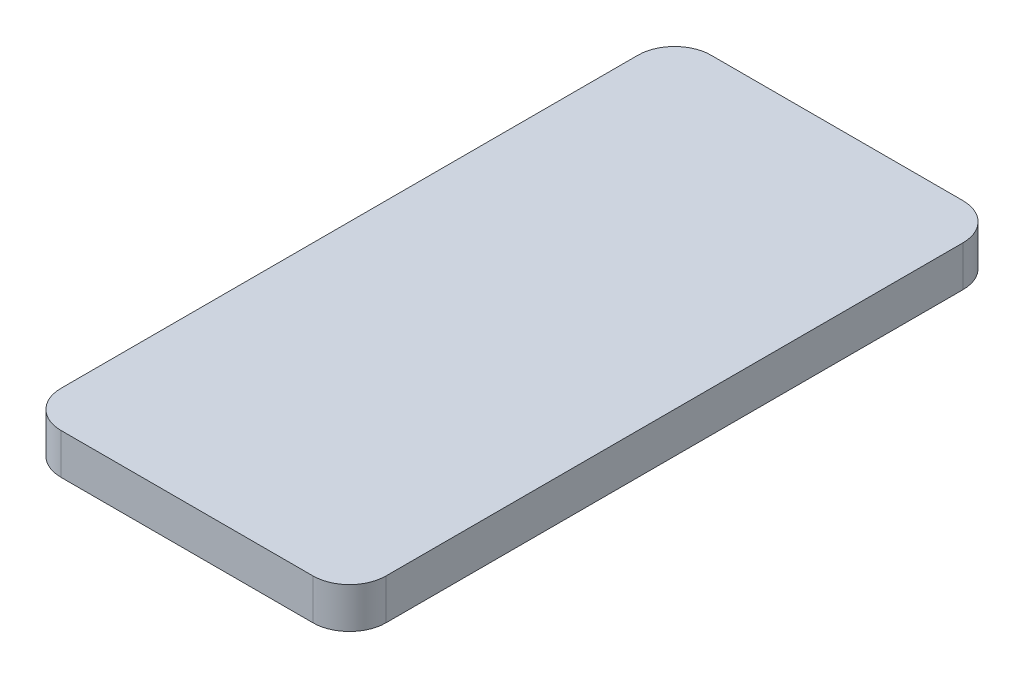
from build123d import *

# Parameters (mm, degrees)
SKETCH_1_W      = 40
SKETCH_1_H      = 80
EXTRUDE_1_DEPTH = 2.5
FILLET_1_R      = 4.5


with BuildPart() as part:
    # 草图1 → 凸台-拉伸1 (new, symmetric)
    with BuildSketch(Plane(origin=(0, 0, 0), x_dir=(1, 0, 0), z_dir=(0, 1, 0))):
        Rectangle(SKETCH_1_W, SKETCH_1_H)
    extrude(amount=EXTRUDE_1_DEPTH, both=True)

    # 圆角1
    fillet_1_edges = [part.edges().sort_by_distance(p)[0] for p in [
        (20, 0, 40),
        (-20, 0, 40),
        (-20, 0, -40),
        (20, 0, -40),
    ]]
    fillet(fillet_1_edges, radius=FILLET_1_R)


solid = part.part
